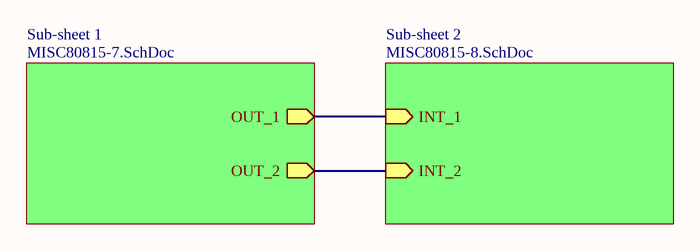
[diagram p0: MISC80815-6.SchDoc]
# Altium project MISC80815.PrjPcb
3 sheets, 22 parts. Net scope: hierarchical (ports join the sheet entries above them; power ports are global).
Board file: MISC80815.PcbDoc
Sheets:
  MISC80815-6.SchDoc
    Sub-sheet 1 = MISC80815-7.SchDoc
    Sub-sheet 2 = MISC80815-8.SchDoc

## Sheet MISC80815-6.SchDoc
size A4

### Sub-sheets
Sub-sheet 1 = MISC80815-7.SchDoc: OUT_1 (out), OUT_2 (out)
Sub-sheet 2 = MISC80815-8.SchDoc: INT_1 (in), INT_2 (in)

### Nets
NetP1_2: sheet Sub-sheet 1/OUT_2, sheet Sub-sheet 2/INT_2
NetR2_2: sheet Sub-sheet 1/OUT_1, sheet Sub-sheet 2/INT_1

## Sheet MISC80815-7.SchDoc
size A4
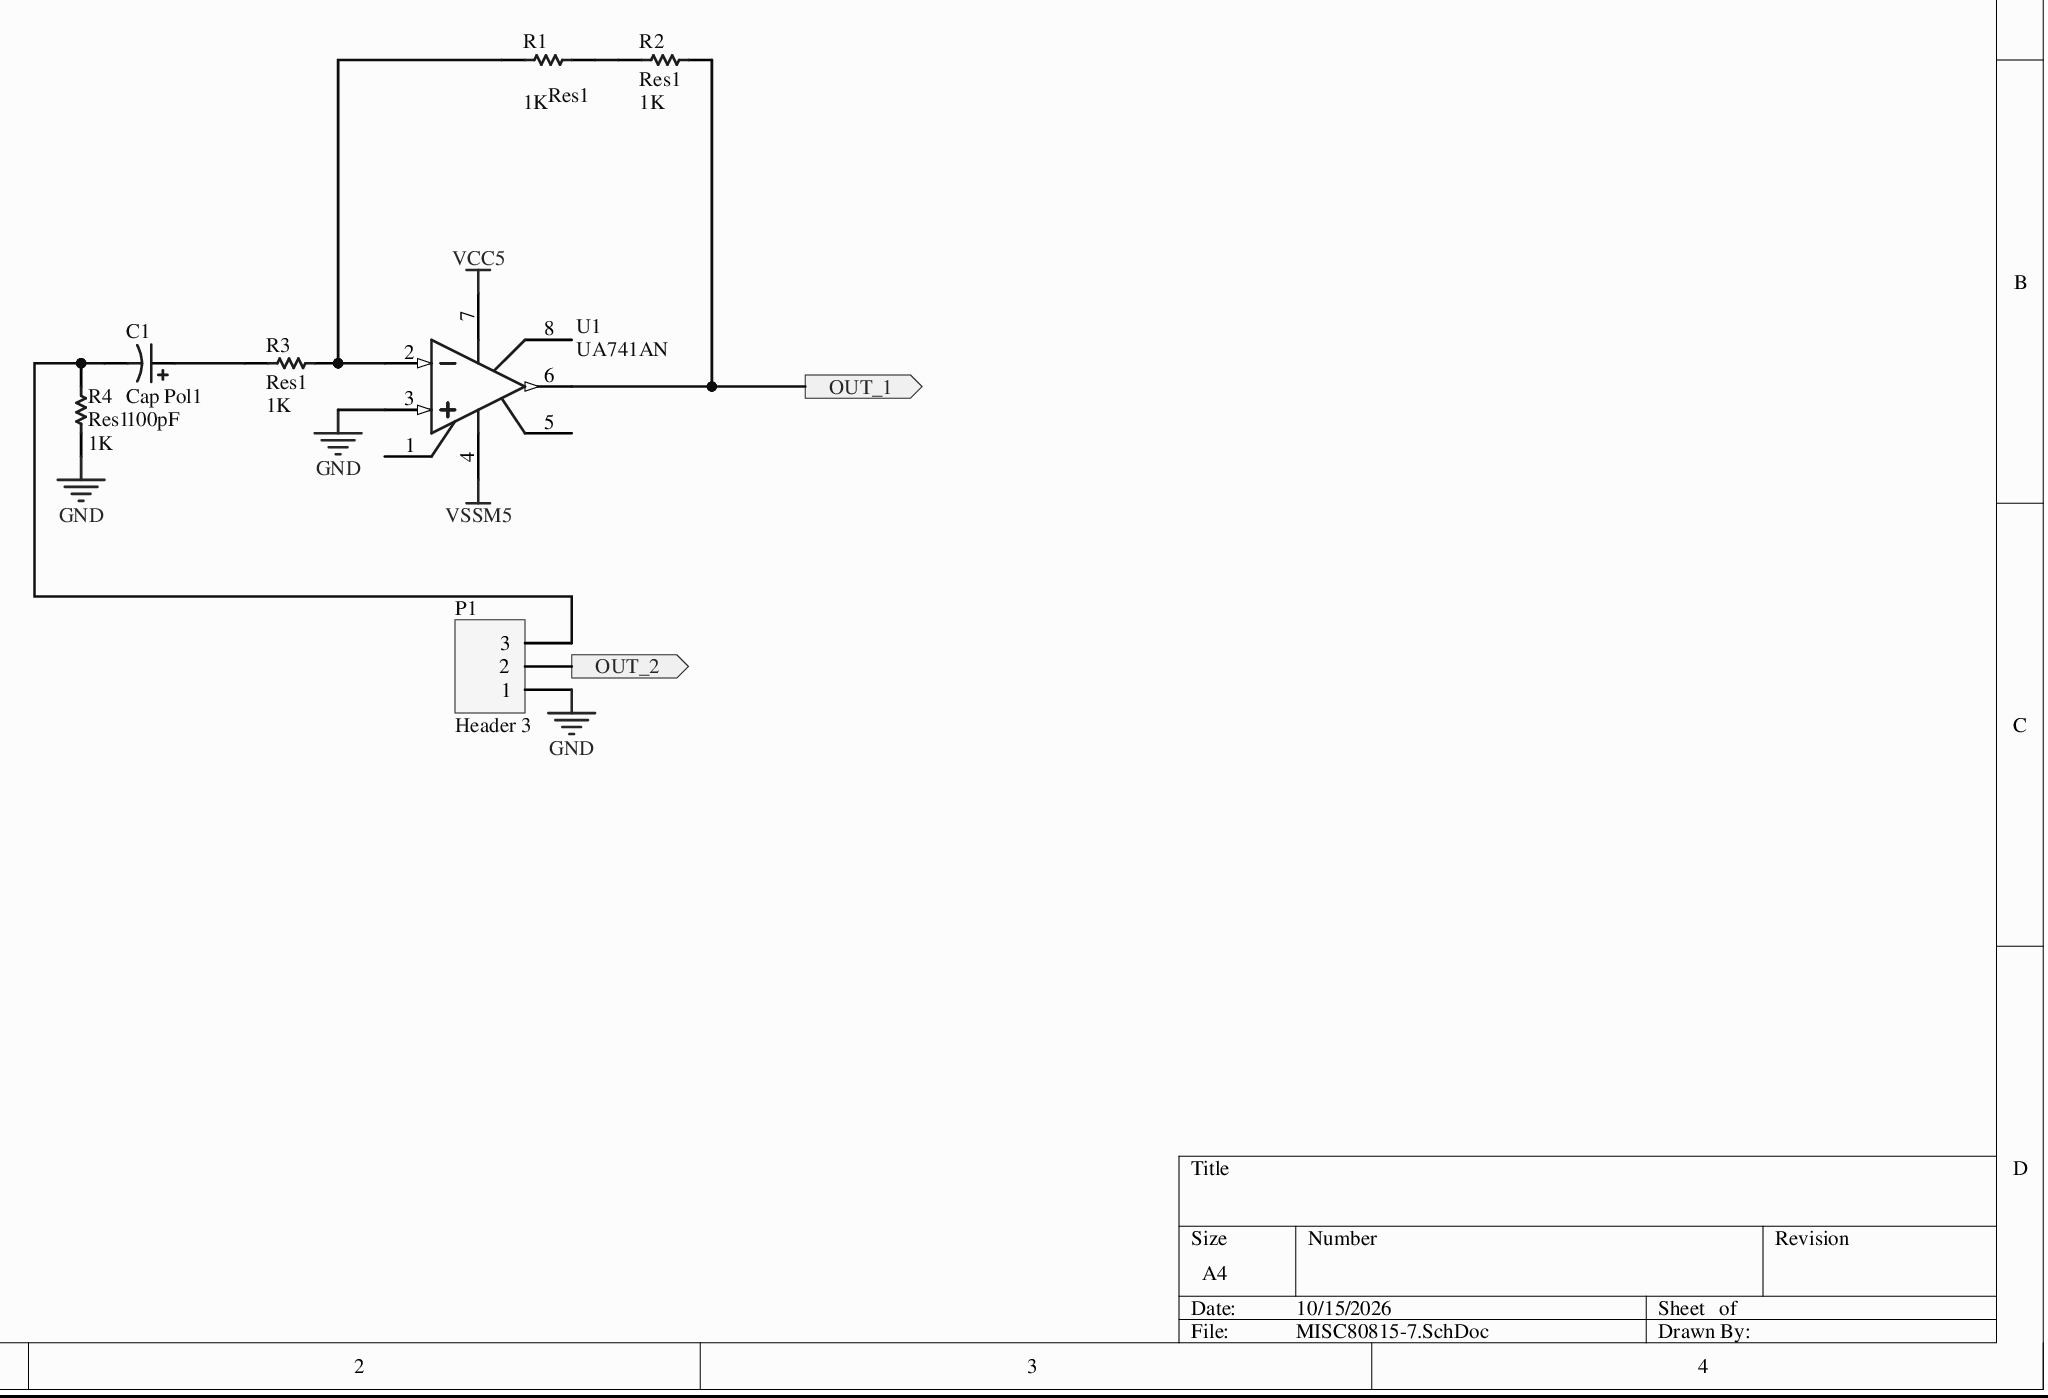
[diagram p1: MISC80815-7.SchDoc]

### Parts
C1  Cap Pol1  value 100pF  [RB7.6-15]
P1  Header 3  [HDR1X3]
R1  Res1  value 1K  [AXIAL-0.3]
R2  Res1  value 1K  [AXIAL-0.3]
R3  Res1  value 1K  [AXIAL-0.3]
R4  Res1  value 1K  [AXIAL-0.3]
U1  UA741AN  [DIP-8]

### Ports
OUT_1 (out), OUT_2 (out)

### Nets
GND: P1.1 R4.1 U1.3(IN+)
VCC5: U1.7(V+)
VSSM5: U1.4(V-)
NetC1_1: C1.1 R3.1
NetC1_2: C1.2 P1.3 R4.2
NetP1_2: P1.2 ; port OUT_2
NetR1_1: R1.1 R3.2 U1.2(IN-)
NetR1_2: R1.2 R2.1
NetR2_2: R2.2 U1.6(OUT) ; port OUT_1

Not connected (* = marked no-connect by the designer): U1 1(OS_NULL) 5(OS_NULL) 8(NC)

### Library data of the parts
C1 = Cap Pol1: Polarized Capacitor (Radial); Published: 8-Jun-2000; LatestRevisionDate: 17-Jul-2002; LatestRevisionNote: Re-released for DXP Platform.; PackageReference: RB7.6-15; PackageDescription: Polarized Capacitor (Radial); 2 Leads; Publisher: Altium Limited
P1 = Header 3: Header, 3-Pin; LatestRevisionDate: 17-Jul-2002; LatestRevisionNote: Re-released for DXP Platform.; Publisher: Altium Limited
R1-R4 = Res1: Resistor; Published: 8-Jun-2000; LatestRevisionDate: 17-Jul-2002; LatestRevisionNote: Re-released for DXP Platform.; PackageReference: AXIAL-0.3; PackageDescription: Axial Device, Thru-Hole; 2 Leads; 0.3 in Pin Spacing; Publisher: Altium Limited
U1 = UA741AN: General-Purpose Single Operational Amplifier; Published: 24-Aug-2001; LatestRevisionDate: 06-Jun-2005; LatestRevisionNote: Stylized 3D Model Added.; DatasheetVersion: Oct-1997; PackageReference: DIP8; PackageDescription: DIP; 8 Leads; Row Spacing 7.62 mm; Pitch 2.54 mm; Code_JEDEC: MO-001-AN; ComponentLink1Description: Manufacturer Link; ComponentLink2Description: Datasheet; ComponentLink2URL: example.com/ds/5304/ua741.pdf; Publisher: Altium Limited

## Sheet MISC80815-8.SchDoc
size A4
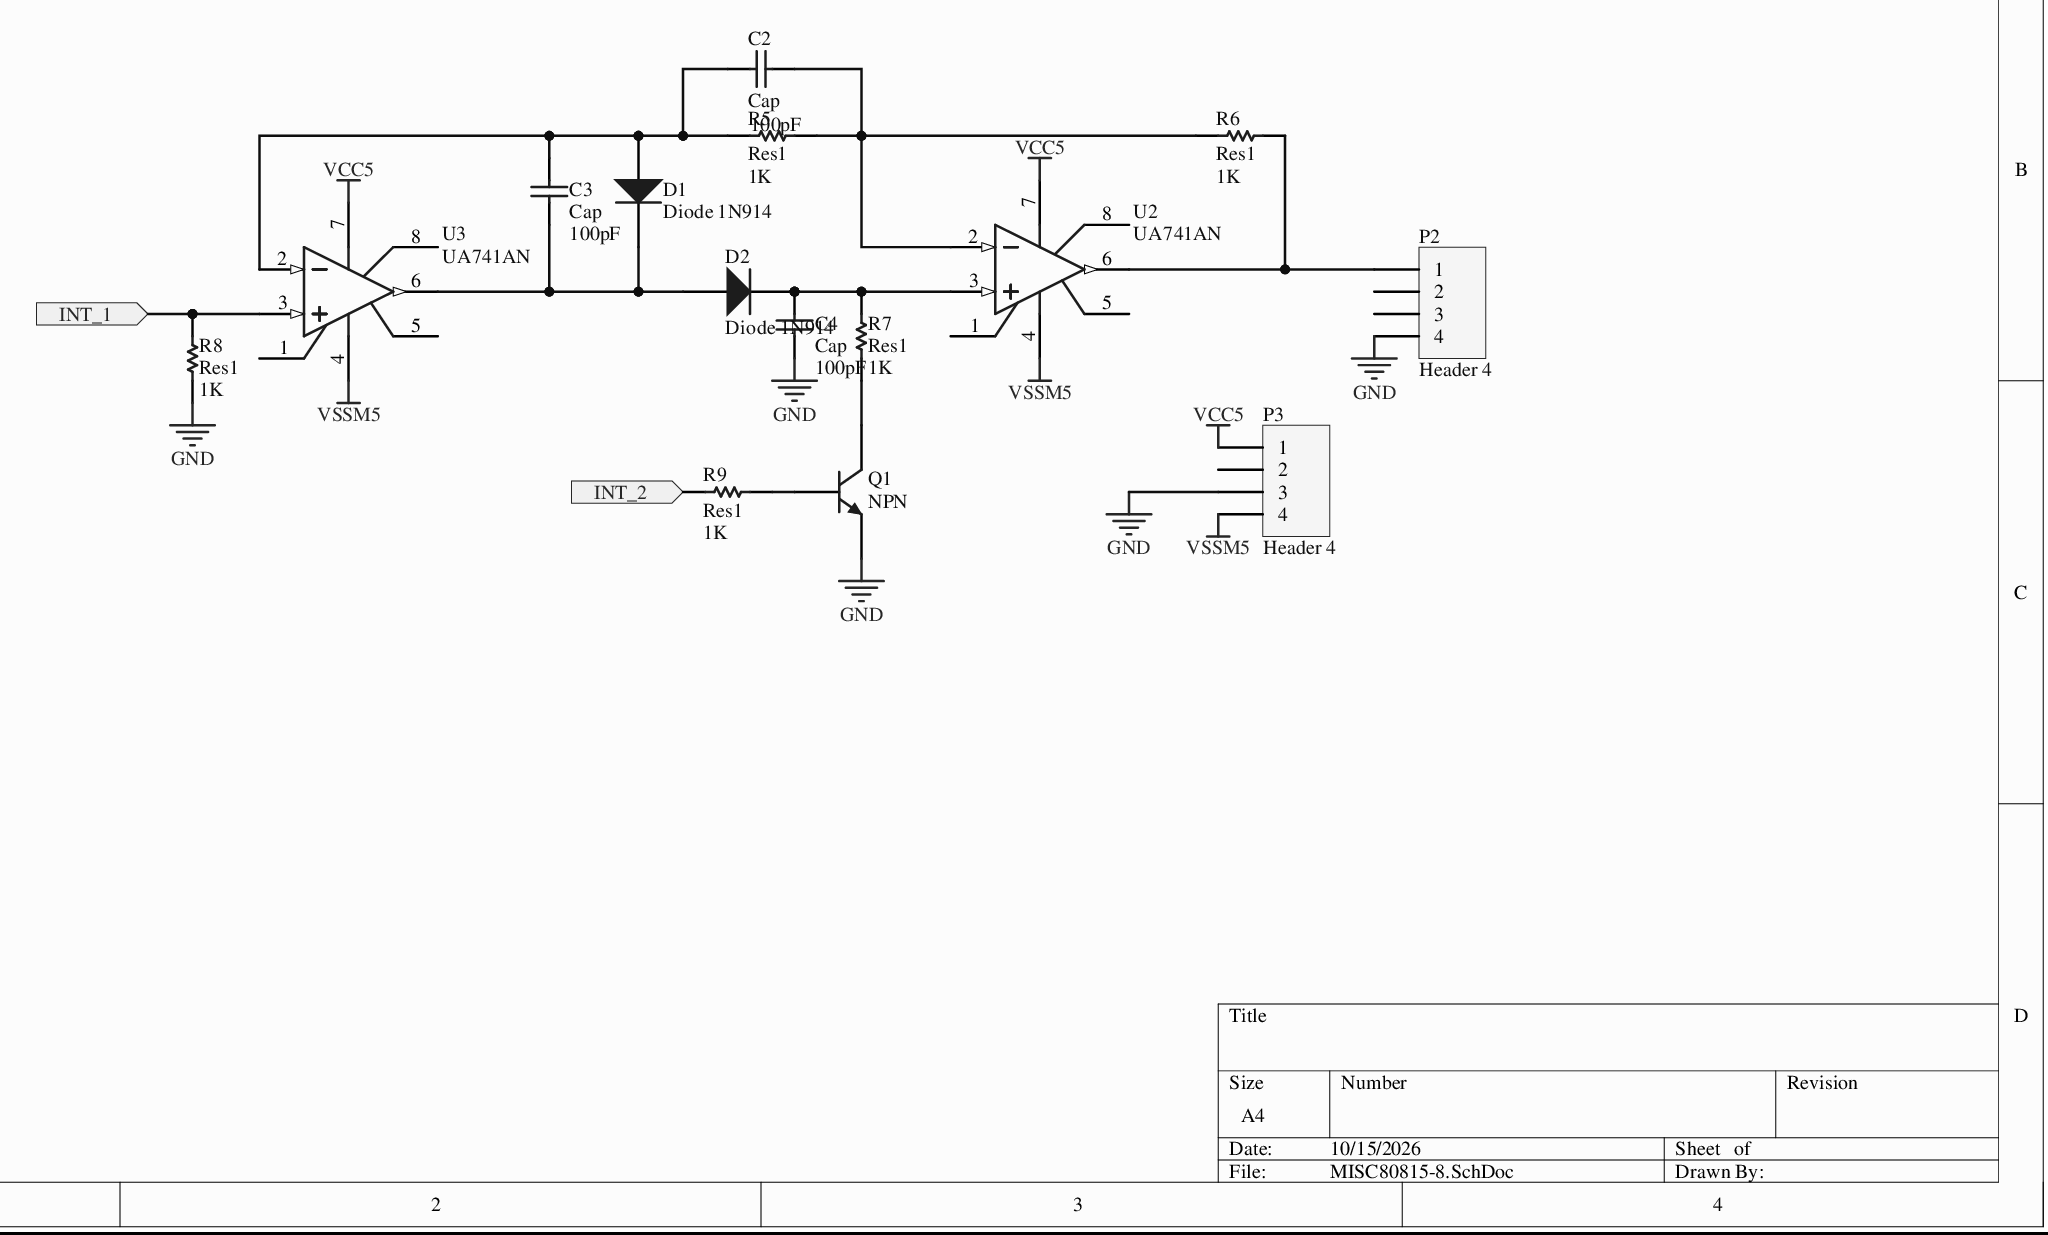
[diagram p2: MISC80815-8.SchDoc]

### Parts
C2  Cap  value 100pF  [RAD-0.3]
C3  Cap  value 100pF  [RAD-0.3]
C4  Cap  value 100pF  [RAD-0.3]
D1  Diode 1N914  [DO-35]
D2  Diode 1N914  [DO-35]
P2  Header 4  [HDR1X4]
P3  Header 4  [HDR1X4]
Q1  NPN  [TO-226-AA]
R5  Res1  value 1K  [AXIAL-0.3]
R6  Res1  value 1K  [AXIAL-0.3]
R7  Res1  value 1K  [AXIAL-0.3]
R8  Res1  value 1K  [AXIAL-0.3]
R9  Res1  value 1K  [AXIAL-0.3]
U2  UA741AN  [DIP-8]
U3  UA741AN  [DIP-8]

### Ports
INT_1 (in), INT_2 (in)

### Nets
GND: C4.2 P2.4 P3.3 Q1.3(E) R8.1
VCC5: P3.1 U2.7(V+) U3.7(V+)
VSSM5: P3.4 U2.4(V-) U3.4(V-)
NetC2_1: C2.1 R5.2 R6.1 U2.2(IN-)
NetC2_2: C2.2 C3.2 D1.1(A) R5.1 U3.2(IN-)
NetC3_1: C3.1 D1.2(K) D2.1(A) U3.6(OUT)
NetC4_1: C4.1 D2.2(K) R7.1 U2.3(IN+)
NetP1_2: R9.2 ; port INT_2
NetP2_1: P2.1 R6.2 U2.6(OUT)
NetQ1_1: Q1.1(C) R7.2
NetQ1_2: Q1.2(B) R9.1
NetR2_2: R8.2 U3.3(IN+) ; port INT_1

Not connected (* = marked no-connect by the designer): P2 2 3; P3 2; U2 1(OS_NULL) 5(OS_NULL) 8(NC); U3 1(OS_NULL) 5(OS_NULL) 8(NC)

### Library data of the parts
C2-C4 = Cap: Capacitor; Published: 8-Jun-2000; LatestRevisionDate: 17-Jul-2002; LatestRevisionNote: Re-released for DXP Platform.; PackageReference: RAD-0.3; PackageDescription: Radial Cap, Thru-Hole; 2 Leads; 0.3 in Pin Spacing; Publisher: Altium Limited
D1 D2 = Diode 1N914: High Conductance Fast Diode; Published: 8-Jun-2000; LatestRevisionDate: 17-Jul-2002; LatestRevisionNote: Re-released for DXP Platform.; DatasheetVersion: 1997; PackageReference: DO-35; PackageDescription: Diode, Axial; Body 3.8 x 1.9 mm (LxDia. max), Lead Dia. 0.53 mm (max); Code_JEDEC: DO-204-AH; ComponentLink1Description: Manufacturer Link; ComponentLink2Description: Datasheet; ComponentLink2URL: example.com/ds/1N%2F1N4448.pdf; Publisher: Altium Limited
P2 P3 = Header 4: Header, 4-Pin; LatestRevisionDate: 17-Jul-2002; LatestRevisionNote: Re-released for DXP Platform.; Publisher: Altium Limited
Q1 = NPN: NPN Bipolar Transistor; Published: 8-Jun-2000; LatestRevisionDate: 17-Jul-2002; LatestRevisionNote: Re-released for DXP Platform.; PackageReference: TO-226-AA; PackageDescription: TO, Flat Index; 3 In-Line, Axial Leads; Body Dia. 4.8mm; Leads 0.55 x 0.51 mm (max); Code_JEDEC: TO-226-AA; Publisher: Altium Limited
R5-R9 = Res1: Resistor; Published: 8-Jun-2000; LatestRevisionDate: 17-Jul-2002; LatestRevisionNote: Re-released for DXP Platform.; PackageReference: AXIAL-0.3; PackageDescription: Axial Device, Thru-Hole; 2 Leads; 0.3 in Pin Spacing; Publisher: Altium Limited
U2 U3 = UA741AN: as U1 on sheet MISC80815-7; Published: 24-Aug-2001; LatestRevisionDate: 06-Jun-2005; LatestRevisionNote: Stylized 3D Model Added.; DatasheetVersion: Oct-1997; PackageReference: DIP8; PackageDescription: DIP; 8 Leads; Row Spacing 7.62 mm; Pitch 2.54 mm; Code_JEDEC: MO-001-AN; ComponentLink1Description: Manufacturer Link; ComponentLink2Description: Datasheet; ComponentLink2URL: example.com/ds/5304/ua741.pdf; Publisher: Altium Limited

## Nets that join several sheets
GND: MISC80815-7 (P1.1 R4.1 U1.3), MISC80815-8 (5 pins)
VCC5: MISC80815-7 (U1.7), MISC80815-8 (P3.1 U2.7 U3.7)
VSSM5: MISC80815-7 (U1.4), MISC80815-8 (P3.4 U2.4 U3.4)
NetP1_2: MISC80815-7 (P1.2), MISC80815-8 (R9.2)
NetR2_2: MISC80815-7 (R2.2 U1.6), MISC80815-8 (R8.2 U3.3)